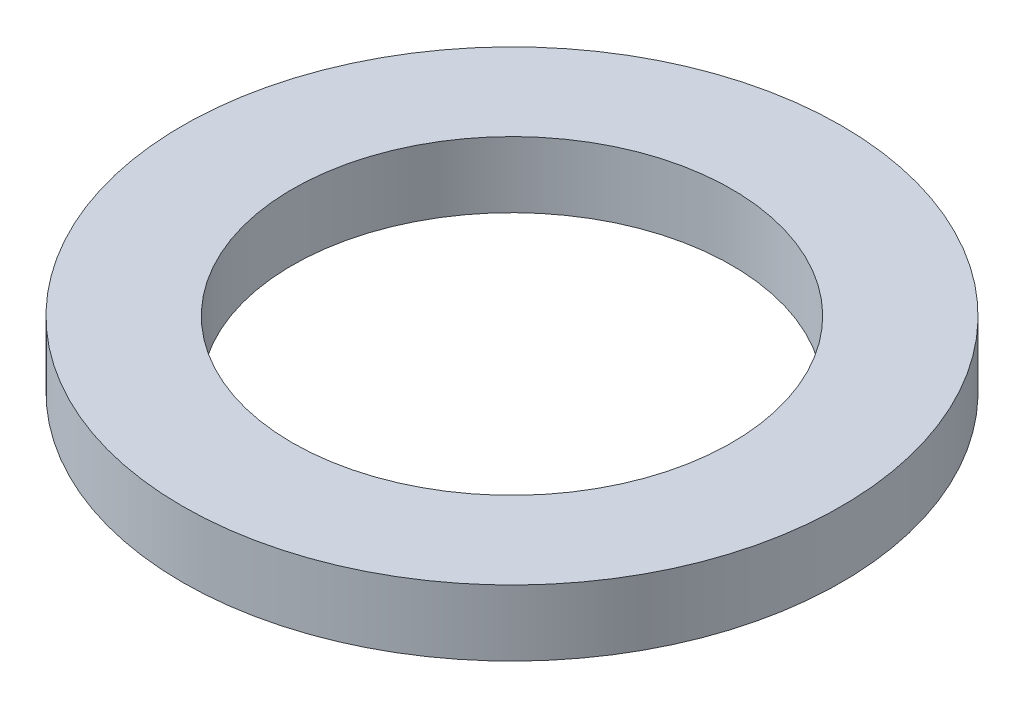
from build123d import *

# Parameters (mm, degrees)
SKETCH1_R           = 15
SKETCH1_R_2         = 10
BOSS_EXTRUDE1_DEPTH = 3


with BuildPart() as part:
    # Sketch1 → Boss-Extrude1 (new body)
    with BuildSketch(Plane(origin=(0, 0, 0), x_dir=(1, 0, 0), z_dir=(0, 1, 0))):
        with Locations(Location((0, 0, 0), (0, 0, 270))):
            Circle(SKETCH1_R)
        with Locations(Location((0, 0, 0), (0, 0, 270))):
            Circle(SKETCH1_R_2, mode=Mode.SUBTRACT)
    extrude(amount=BOSS_EXTRUDE1_DEPTH)


solid = part.part
